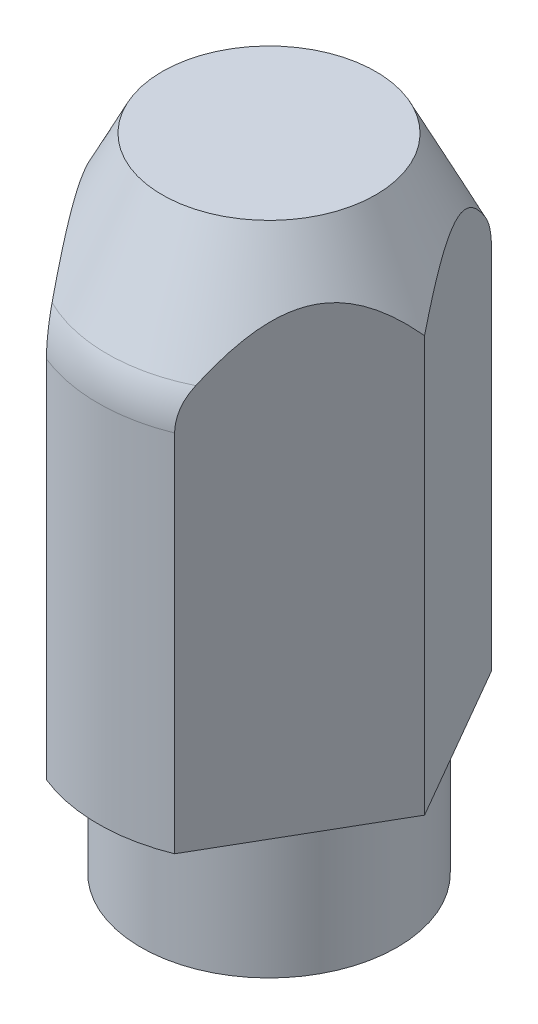
SolidWorks part; units mm, degrees
material "SKD11"
ref_plane "Front Plane" through (0, 0, 0) normal (0, 0, 1) x (1, 0, 0)
ref_plane "Top Plane" through (0, 0, 0) normal (0, 1, 0) x (1, 0, 0)
ref_plane "Right Plane" through (0, 0, 0) normal (1, 0, 0) x (0, 0, -1)
sketch "Sketch1" plane through (0, 0, 0) normal (0, 0, 1) x (1, 0, 0)
  line L0 (0, 0) -> (0, 15)
  line L1 (0, 15) -> (2.5, 15)
  line L2 (4, 12) -> (4, 3)
  line L3 (3, 0) -> (0, 0)
  line L4 (2.5, 15) -> (4, 12)
  line L5 (4, 3) -> (3, 3)
  line L6 (3, 3) -> (3, 0)
  dimension "D1" = 4
  dimension "D2" = 15
  dimension "D3" = 1.5
  dimension "D4" = 3
  dimension "D5" = 3
  dimension "D6" = 3
revolve "Revolve1" add sketch "Sketch1" angle 360 about L0
hole_wizard "M3 Tapped Hole1" positions "Sketch2" profile "Sketch3" tap size "M3" standard "ISO"
sketch "Sketch2" plane through (0, 0, 0) normal (0, -1, 0) x (-1, 0, 0)
  point P0 (0, 0)
sketch "Sketch3" plane through (0, 0, 0) normal (1, 0, 0) x (0, 0, -1)
  line L0 (0, 0) -> (0, 10.7511)
  line L1 (0, 10.7511) -> (1.25, 10)
  line L2 (1.25, 10) -> (1.25, 0)
  line L5 (1.25, 0) -> (0, 0)
  line L10 (0, 10.7511) -> (-1.25, 10) construction
  line L11 (0, -6.35) -> (0, 107.95) construction
  dimension "螺纹孔钻头直径" = 2.5
  dimension "螺纹孔钻头深度" = 10
  dimension "导头角度" = 118
cosmetic thread "Cosmetic thread 1" parameters "D1"=8, "D2"=3
sketch "Sketch4" plane through (0, 15, 0) normal (0, 1, 0) x (1, 0, 0)
  line L0 (-3.6409, 0) -> (3.6409, 0) construction
  line L1 (0, 0) -> (0, 4) construction
  line L2 (-1.5, 3.7081) -> (-3.6409, 0)
  line L3 (-3.6409, 0) -> (-1.5, -3.7081)
  line L4 (1.5, 3.7081) -> (3.6409, 0)
  line L5 (3.6409, 0) -> (1.5, -3.7081)
  circle A0 centre (0, 0) radius 4 construction
  arc A1 (1.5, -3.7081) -> (1.5, 3.7081) centre (0, 0) ccw
  arc A2 (-1.5, 3.7081) -> (-1.5, -3.7081) centre (0, 0) ccw
  dimension "D1" = 3
  dimension "D2" = 60
extrude "Cut-Extrude1" cut sketch "Sketch4" against normal through all
fillet "Fillet1" radius 2 2 edges at (0, 12, -4) (0, 12, 4)
